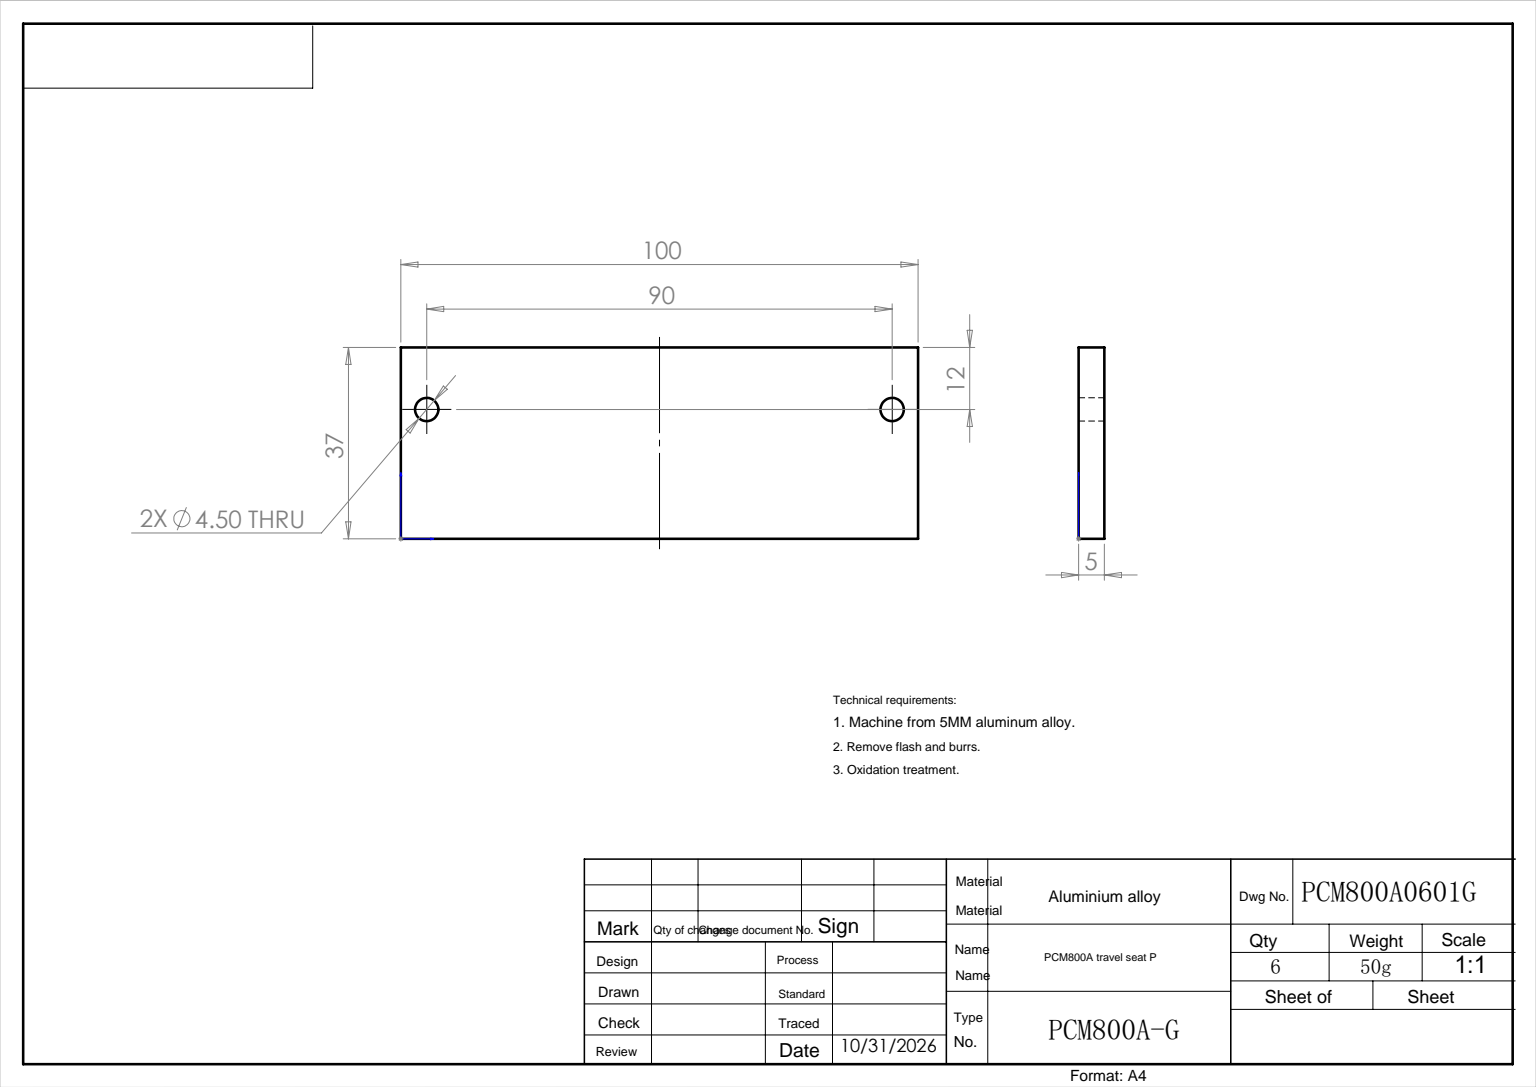
SolidWorks part; units mm, degrees
ref_plane "前视基准面" through (0, 0, 0) normal (0, 0, 1) x (1, 0, 0)
ref_plane "上视基准面" through (0, 0, 0) normal (0, 1, 0) x (1, 0, 0)
ref_plane "右视基准面" through (0, 0, 0) normal (1, 0, 0) x (0, 0, -1)
sketch "草图1" plane through (0, 0, 0) normal (0, 0, 1) x (1, 0, 0)
  line L1 (0, 0) -> (100, 0)
  line L2 (0, 0) -> (0, 37)
  line L3 (0, 37) -> (100, 37)
  line L4 (100, 0) -> (100, 37)
  dimension "D1" = 37
  dimension "D2" = 100
extrude "凸台-拉伸1" add sketch "草图1" along normal blind 5
sketch "草图2" plane through (0, 0, 5) normal (0, 0, 1) x (1, 0, 0)
  line L0 (5, 25) -> (95, 25) construction
  line L2 (50, 37) -> (50, -4.6351) construction
  line L3 (100, 37) -> (0, 37) construction
  line L4 (0, 37) -> (0, 0) construction
  line L5 (100, 0) -> (100, 37) construction
  circle A0 centre (5, 25) radius 2.25
  circle A1 centre (95, 25) radius 2.25
  dimension "D1" = 4.5
  dimension "D2" = 4.5
  dimension "D3" = 5
  dimension "D4" = 5
  dimension "D5" = 12
extrude "切除-拉伸1" cut sketch "草图2" against normal blind 5
